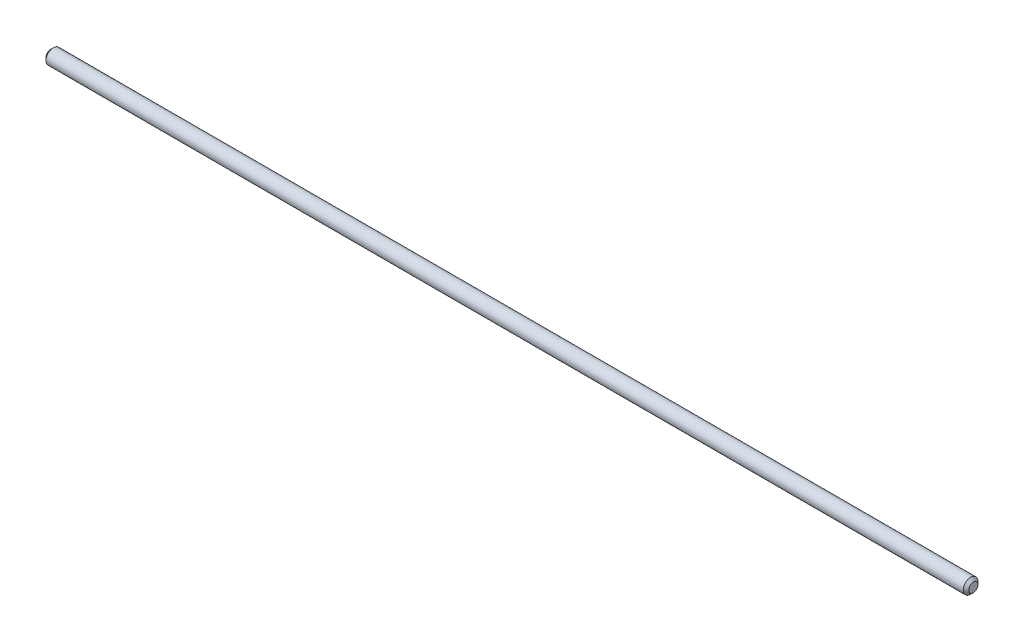
from build123d import *

# Parameters (mm, degrees)
SKETCH1_R           = 4
BOSS_EXTRUDE1_DEPTH = 250
CHAMFER1_SIZE       = 1.5


with BuildPart() as part:
    # Sketch1 → Boss-Extrude1 (new, symmetric)
    with BuildSketch(Plane(origin=(0, 0, 0), x_dir=(0, 0, -1), z_dir=(1, 0, 0))):
        Circle(SKETCH1_R)
    extrude(amount=BOSS_EXTRUDE1_DEPTH, both=True)

    # Chamfer1
    chamfer1_edges = [part.edges().sort_by_distance(p)[0] for p in [
        (-250, 0, 4),
        (250, 0, 4),
    ]]
    chamfer(chamfer1_edges, length=CHAMFER1_SIZE)


solid = part.part
